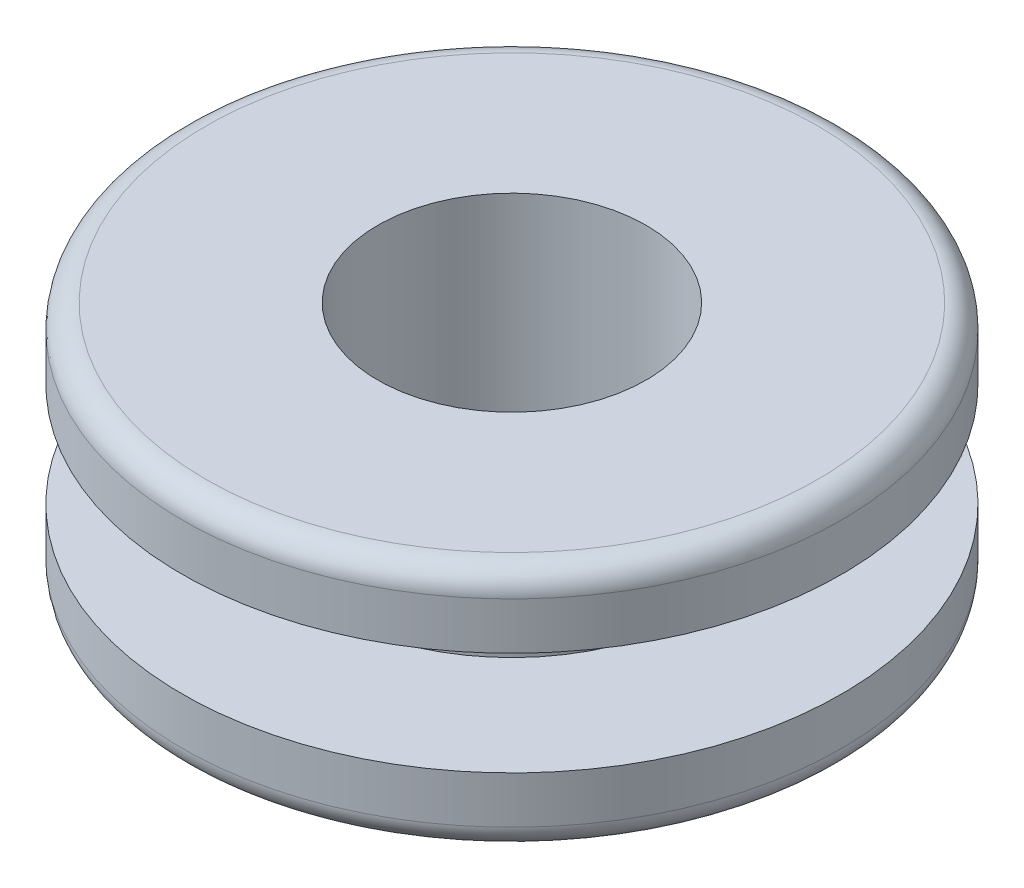
from build123d import *


with BuildPart() as part:
    # 草图1 → 旋转1 (revolve)
    with BuildSketch(Plane.XY, mode=Mode.PRIVATE) as revolve_1_sk:
        with BuildLine():
            Line((2.85, 5.2), (6.5, 5.2))
            ThreePointArc((6.5, 5.2), (6.853553391, 5.053553391), (7, 4.7))
            Line((7, 4.7), (7, 3.7))
            Line((7, 3.7), (4, 3.7))
            Line((4, 3.7), (4, 1.5))
            Line((4, 1.5), (7, 1.5))
            Line((7, 1.5), (7, 0.5))
            ThreePointArc((7, 0.5), (6.853553391, 0.146446609), (6.5, 0))
            Line((6.5, 0), (2.85, 0))
            Line((2.85, 0), (2.85, 5.2))
        make_face()
    revolve(revolve_1_sk.sketch.rotate(Axis((0, 0, 0), (0, 1, 0)), 90), axis=Axis((0, 0, 0), (0, 1, 0)))


solid = part.part
